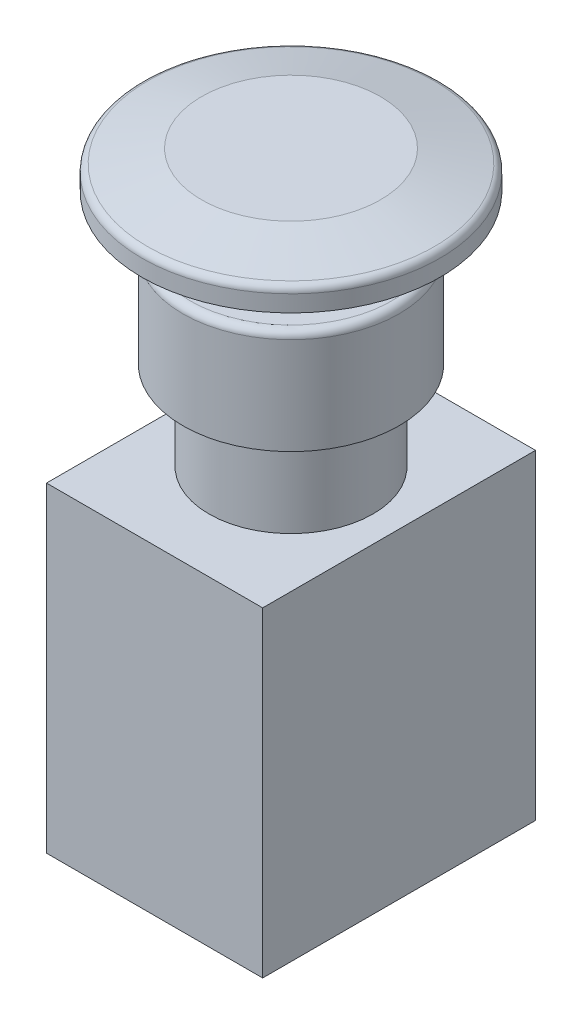
SolidWorks part; units mm, degrees
ref_plane "Front Plane" through (0, 0, 0) normal (0, 0, 1) x (1, 0, 0)
ref_plane "Top Plane" through (0, 0, 0) normal (0, 1, 0) x (1, 0, 0)
ref_plane "Right Plane" through (0, 0, 0) normal (1, 0, 0) x (0, 0, -1)
sketch "Sketch1" plane through (0, 0, 0) normal (0, 1, 0) x (1, 0, 0)
  circle A0 centre (0, 0) radius 14.5
  dimension "D1" = 29
extrude "Boss-Extrude1" add sketch "Sketch1" along normal blind 14
sketch "Sketch2" plane through (0, 14, 0) normal (0, 1, 0) x (1, 0, 0)
  circle A0 centre (0, 0) radius 11
  dimension "D1" = 22
extrude "Boss-Extrude2" add sketch "Sketch2" along normal blind 6
sketch "Sketch3" plane through (0, 20, 0) normal (0, 1, 0) x (1, 0, 0)
  circle A0 centre (0, 0) radius 20
  dimension "D1" = 40
extrude "Boss-Extrude3" add sketch "Sketch3" along normal blind 5
sketch "Sketch4" plane through (0, 0, 0) normal (0, 0, 1) x (1, 0, 0)
  line L0 (0, 0) -> (0, 25) construction
  line L1 (20, 25) -> (-20, 25) construction
  line L2 (-12, 25) -> (-20, 25)
  line L3 (-20, 25) -> (-20, 23)
  line L5 (-20, 23) -> (-12, 25)
  dimension "D1" = 8
  dimension "D2" = 2
revolve "Cut-Revolve1" cut sketch "Sketch4" angle 360 about L0
fillet "Fillet1" radius 1 2 edges at (0, 23, -20) (0, 14, 14.5)
sketch "Sketch5" plane through (0, 0, 0) normal (0, -1, 0) x (1, 0, 0)
  circle A0 centre (0, 0) radius 11
  dimension "D1" = 22
extrude "Boss-Extrude4" add sketch "Sketch5" along normal blind 12
sketch "Sketch6" plane through (0, -12, 0) normal (0, -1, 0) x (1, 0, 0)
  line L1 (-14.5, -18.3) -> (14.5, -18.3)
  line L2 (-14.5, -18.3) -> (-14.5, 18.3)
  line L3 (-14.5, 18.3) -> (14.5, 18.3)
  line L4 (14.5, -18.3) -> (14.5, 18.3)
  line L5 (-14.5, -18.3) -> (14.5, 18.3) construction
  line L6 (-14.5, 18.3) -> (14.5, -18.3) construction
  point P0 (0, 0)
  dimension "D1" = 29
  dimension "D2" = 36.6
extrude "Boss-Extrude5" add sketch "Sketch6" along normal blind 43
